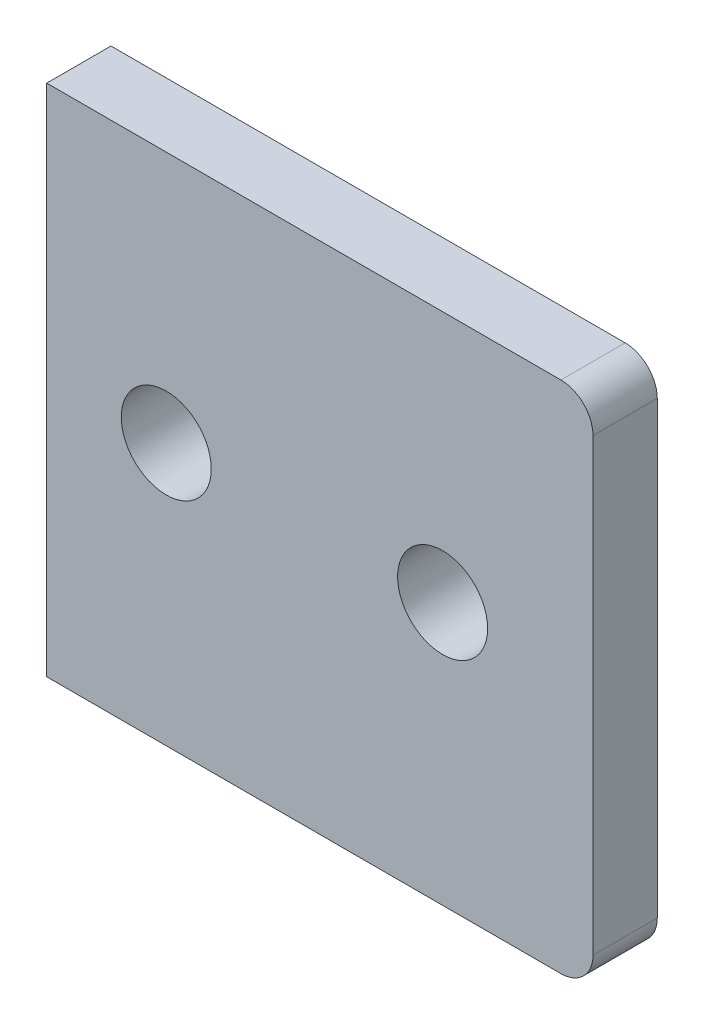
SolidWorks part; units mm, degrees
ref_plane "前视基准面" through (0, 0, 0) normal (0, 0, 1) x (1, 0, 0)
ref_plane "上视基准面" through (0, 0, 0) normal (0, 1, 0) x (1, 0, 0)
ref_plane "右视基准面" through (0, 0, 0) normal (1, 0, 0) x (0, 0, -1)
sketch "草图1" plane through (0, 0, 0) normal (0, 0, 1) x (1, 0, 0)
  line L1 (-42.5, 40) -> (37.5, 40)
  line L2 (-42.5, 40) -> (-42.5, -40)
  line L3 (-42.5, -40) -> (37.5, -40)
  line L4 (42.5, 35) -> (42.5, -35)
  line L5 (-42.5, 40) -> (42.5, -40) construction
  line L6 (-42.5, -40) -> (42.5, 40) construction
  arc A2 (37.5, -40) -> (42.5, -35) centre (37.5, -35) ccw
  arc A3 (37.5, 40) -> (42.5, 35) centre (37.5, 35) cw
  point P0 (0, 0)
  dimension "D6" = 5
  dimension "D1" = 85
  dimension "D2" = 80
extrude "凸台-拉伸1" add sketch "草图1" along normal blind 10
hole_wizard "Ø14.0 (14) 直径孔1" positions "草图2" profile "草图3" hole size "Ø14.0" standard "GB"
sketch "草图2" plane through (0, 0, 10) normal (0, 0, 1) x (1, 0, 0)
  line L0 (27.1, 7.8) -> (11.1, 7.8) construction
  line L1 (-16.9, 8.8) -> (-16.9, -7.2) construction
  arc A0 (11.1, 7.8) -> (10.6293, -6.1842) centre (11.1, 0.8) ccw construction
  point P0 (19.1, 0.8)
  point P2 (-23.9, 0.8)
  dimension "D1" = 8
  dimension "D2" = 7
  dimension "D3" = 7
  dimension "D4" = 8
sketch "草图3" plane through (19.1, 0.8, 10) normal (1, 0, 0) x (0, -1, 0)
  line L0 (0, 0) -> (0, 24)
  line L1 (0, 24) -> (7, 19.794)
  line L2 (7, 19.794) -> (7, 0)
  line L5 (7, 0) -> (0, 0)
  line L10 (0, 24) -> (-7, 19.794) construction
  line L11 (0, -6.35) -> (0, 107.95) construction
  dimension "孔直径" = 14
  dimension "孔深度" = 24
  dimension "导头角度" = 118
